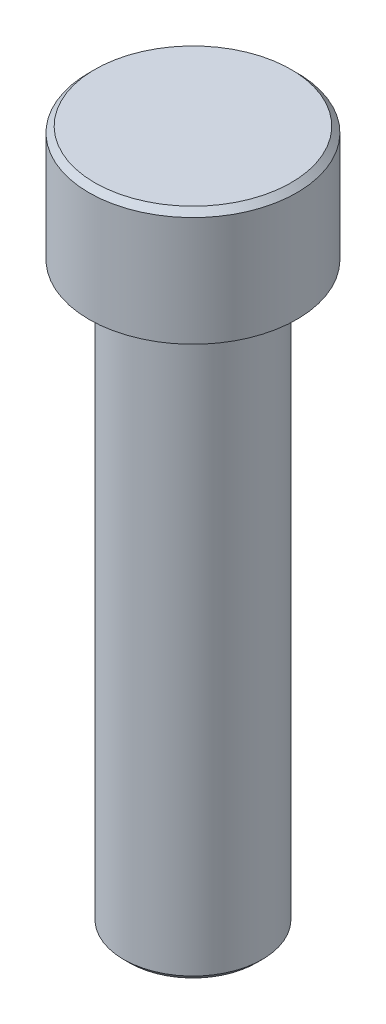
SolidWorks part; units mm, degrees
ref_plane "前视基准面" through (0, 0, 0) normal (0, 0, 1) x (1, 0, 0)
ref_plane "上视基准面" through (0, 0, 0) normal (0, 1, 0) x (1, 0, 0)
ref_plane "右视基准面" through (0, 0, 0) normal (1, 0, 0) x (0, 0, -1)
other "Configuration Table"
sketch "草图1" plane through (0, 0, 0) normal (0, 1, 0) x (1, 0, 0)
  circle A0 centre (0, 0) radius 6
  dimension "D1" = 12
extrude "凸台-拉伸1" add sketch "草图1" along normal mid plane 50 contours A0
sketch "草图2" plane through (0, 25, 0) normal (0, 1, 0) x (1, 0, 0)
  circle A0 centre (0, 0) radius 9
  dimension "D1" = 18
extrude "凸台-拉伸2" add sketch "草图2" along normal blind 10 contours A0
chamfer "倒角1" distance 0.5 angle 45 2 edges at (0, -25, 6) (0, 35, 9)
